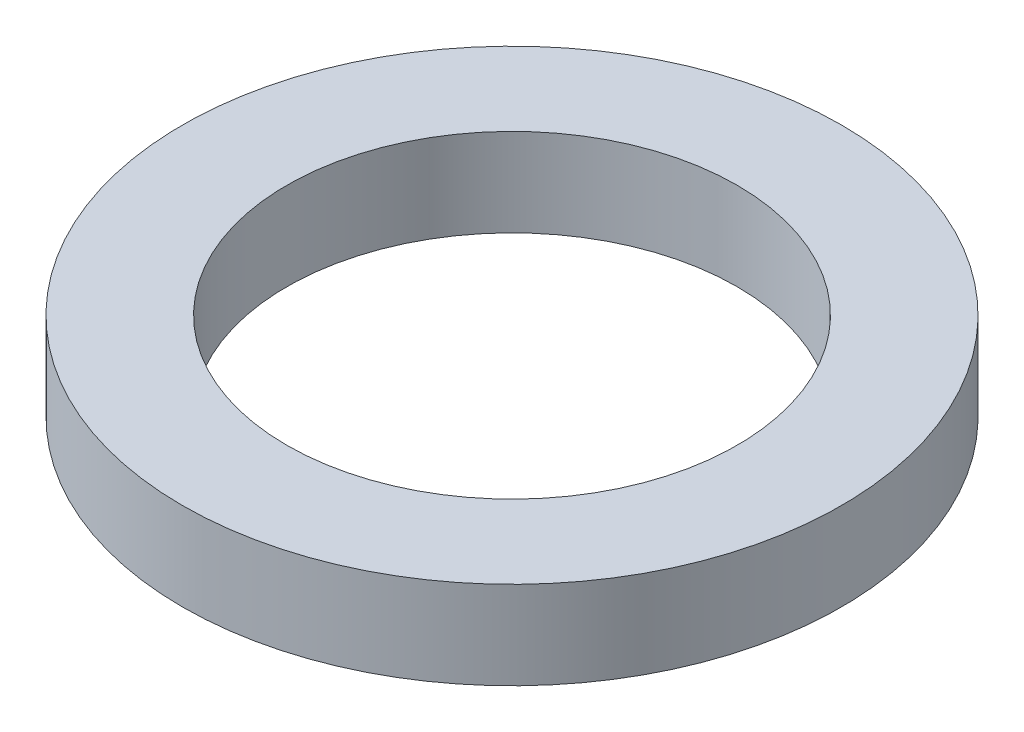
from build123d import *

# Parameters (mm, degrees)
SKETCH1_R           = 6
SKETCH1_R_2         = 4.1
BOSS_EXTRUDE1_DEPTH = 1.6


with BuildPart() as part:
    # Sketch1 → Boss-Extrude1 (new body)
    with BuildSketch(Plane(origin=(0, 0, 0), x_dir=(1, 0, 0), z_dir=(0, 1, 0))):
        with Locations(Location((0, 0, 0), (0, 0, 270))):
            Circle(SKETCH1_R)
        with Locations(Location((0, 0, 0), (0, 0, 270))):
            Circle(SKETCH1_R_2, mode=Mode.SUBTRACT)
    extrude(amount=BOSS_EXTRUDE1_DEPTH)


solid = part.part
